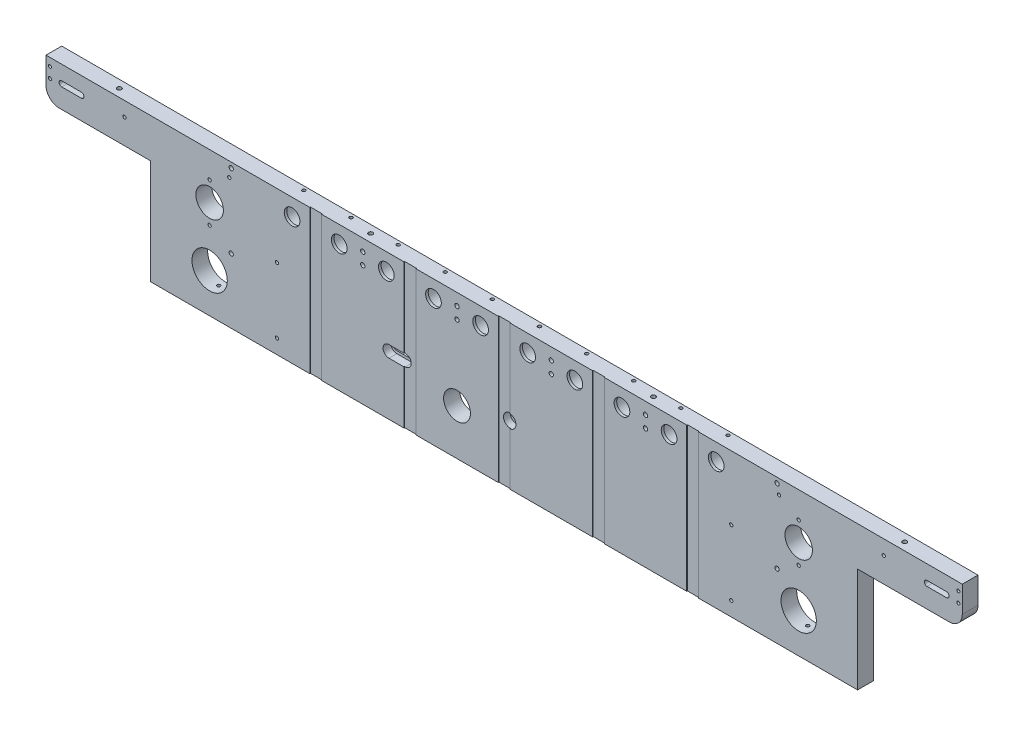
from build123d import *

# Parameters (mm, degrees)
EXTRUDE_1_DEPTH           = 12
FILLET_1_R                = 10
SKETCH_3_R                = 10.5
SKETCH_3_R_2              = 13.5
SKETCH_3_R_3              = 10.25
CUT_EXTRUDE_2_DEPTH       = 368.074924232
SKETCH_7_R                = 7.5
CUT_EXTRUDE_3_DEPTH       = 10
SKETCH_8_R                = 5.5
CUT_EXTRUDE_4_DEPTH       = 368.01498607
CUT_EXTRUDE_5_DEPTH       = 368.074924232
HOLE_WIZARD_M3_2_REACH    = 369.075
HOLE_WIZARD_M3_2_BORE_R   = 1.25
HOLE_WIZARD_M3_3_D        = 2.5
HOLE_WIZARD_1_D           = 5.5
HOLE_WIZARD_1_CBORE_D     = 10
HOLE_WIZARD_1_CBORE_DEPTH = 5.7
CUT_EXTRUDE_7_DEPTH       = 368.074924265
CUT_EXTRUDE_8_DEPTH       = 6
SKETCH_35_W               = 9
SKETCH_35_H               = 0.5
CUT_EXTRUDE_9_DEPTH       = 368.074924265
HOLE_WIZARD_M4_2_D        = 3.3
HOLE_WIZARD_M4_2_DEPTH    = 12
HOLE_WIZARD_M4_2_TIP      = 0.991420021
HOLE_WIZARD_M3_4_REACH    = 369.075
HOLE_WIZARD_M3_4_BORE_R   = 1.25
HOLE_WIZARD_M3_5_D        = 2.5
HOLE_WIZARD_M4_3_D        = 3.3
PATTERN_LINEAR_1_COUNT    = 4
PATTERN_LINEAR_1_PITCH    = 72
HOLE_WIZARD_M4_4_D        = 3.3
HOLE_WIZARD_M4_4_DEPTH    = 12
HOLE_WIZARD_M4_4_TIP      = 0.991420021
HOLE_WIZARD_2_D           = 2.4
HOLE_WIZARD_2_CBORE_D     = 4.3
HOLE_WIZARD_2_CBORE_DEPTH = 2.3
HOLE_WIZARD_3_D           = 2.4
HOLE_WIZARD_3_CBORE_D     = 4.3
HOLE_WIZARD_3_CBORE_DEPTH = 2.3
HOLE_WIZARD_4_D           = 12
HOLE_WIZARD_4_CBORE_D     = 16
HOLE_WIZARD_4_CBORE_DEPTH = 10
HOLE_WIZARD_M3_6_D        = 2.5


with BuildPart() as part:
    # 草图1 → 凸台-拉伸1 (new body)
    with BuildSketch(Plane.XY):
        Polygon((-350, -30), (-270, -30), (-270, -110), (270, -110), (270, -30), (350, -30), (350, 0), (-350, 0), align=None)
    extrude(amount=EXTRUDE_1_DEPTH)

    # 圆角1
    fillet_1_edges = [part.edges().sort_by_distance(p)[0] for p in [
        (350, -30, 6),
        (-350, -30, 6),
    ]]
    fillet(fillet_1_edges, radius=FILLET_1_R)

    # 草图3 → 切除-拉伸2 (cut, through all)
    with BuildSketch(Plane(origin=(0, 0, 0), x_dir=(-1, 0, 0), z_dir=(0, 0, -1))):
        with Locations((-225, -35)):
            Circle(SKETCH_3_R)
        with Locations((-225, -80)):
            Circle(SKETCH_3_R_2)
        with Locations(Location((225, -80, 0), (0, 0, 180))):
            Circle(SKETCH_3_R_2)
        with Locations(Location((225, -35, 0), (0, 0, 180))):
            Circle(SKETCH_3_R)
        with Locations((36, -75)):
            Circle(SKETCH_3_R_3)
    extrude(amount=-CUT_EXTRUDE_2_DEPTH, mode=Mode.SUBTRACT)

    # 草图7 → 切除-拉伸3 (cut)
    with BuildSketch(Plane(origin=(0, 0, 0), x_dir=(-1, 0, 0), z_dir=(0, 0, -1))):
        with Locations((-162, -13)):
            Circle(SKETCH_7_R)
        with Locations((-126, -13)):
            Circle(SKETCH_7_R)
        with Locations((-90, -13)):
            Circle(SKETCH_7_R)
        with Locations((-54, -13)):
            Circle(SKETCH_7_R)
        with Locations((-18, -13)):
            Circle(SKETCH_7_R)
        with Locations((18, -13)):
            Circle(SKETCH_7_R)
        with Locations((54, -13)):
            Circle(SKETCH_7_R)
        with Locations((90, -13)):
            Circle(SKETCH_7_R)
        with Locations((126, -13)):
            Circle(SKETCH_7_R)
        with Locations((162, -13)):
            Circle(SKETCH_7_R)
    extrude(amount=-CUT_EXTRUDE_3_DEPTH, mode=Mode.SUBTRACT)

    # 草图8 → 切除-拉伸4 (cut, through all)
    with BuildSketch(Plane(origin=(0, 0, 10), x_dir=(-1, 0, 0), z_dir=(0, 0, -1))):
        with Locations((-162, -13)):
            Circle(SKETCH_8_R)
        with Locations((-126, -13)):
            Circle(SKETCH_8_R)
        with Locations((-90, -13)):
            Circle(SKETCH_8_R)
        with Locations((-54, -13)):
            Circle(SKETCH_8_R)
        with Locations((-18, -13)):
            Circle(SKETCH_8_R)
        with Locations((18, -13)):
            Circle(SKETCH_8_R)
        with Locations((54, -13)):
            Circle(SKETCH_8_R)
        with Locations((90, -13)):
            Circle(SKETCH_8_R)
        with Locations((126, -13)):
            Circle(SKETCH_8_R)
        with Locations((162, -13)):
            Circle(SKETCH_8_R)
    extrude(amount=-CUT_EXTRUDE_4_DEPTH, mode=Mode.SUBTRACT)

    # 草图9 → 切除-拉伸5 (cut, through all)
    with BuildSketch(Plane(origin=(0, 0, 0), x_dir=(-1, 0, 0), z_dir=(0, 0, -1))):
        with BuildLine():
            Line((-338, -11), (-323, -11))
            ThreePointArc((-323, -11), (-321, -13), (-323, -15))
            Line((-323, -15), (-338, -15))
            ThreePointArc((-338, -15), (-340, -13), (-338, -11))
        make_face()
        with BuildLine():
            Line((338, -11), (323, -11))
            ThreePointArc((323, -11), (321, -13), (323, -15))
            Line((323, -15), (338, -15))
            ThreePointArc((338, -15), (340, -13), (338, -11))
        make_face()
    extrude(amount=-CUT_EXTRUDE_5_DEPTH, mode=Mode.SUBTRACT)

    # M3 螺纹孔2 bore → M3 螺纹孔2 (cut, up to next)
    with BuildSketch(Plane(origin=(0, -110, 0), x_dir=(-1, 0, 0), z_dir=(0, -1, 0)), mode=Mode.PRIVATE) as hole_wizard_m3_2_sk1:
        with Locations((225, -5)):
            Circle(HOLE_WIZARD_M3_2_BORE_R)
    hole_wizard_m3_2_tool1 = extrude(hole_wizard_m3_2_sk1.sketch, amount=-HOLE_WIZARD_M3_2_REACH, mode=Mode.PRIVATE) & part.part
    # M3 螺纹孔2 bore → M3 螺纹孔2 (cut, up to next)
    with BuildSketch(Plane(origin=(0, -110, 0), x_dir=(-1, 0, 0), z_dir=(0, -1, 0)), mode=Mode.PRIVATE) as hole_wizard_m3_2_sk2:
        with Locations((-225, -5)):
            Circle(HOLE_WIZARD_M3_2_BORE_R)
    hole_wizard_m3_2_tool2 = extrude(hole_wizard_m3_2_sk2.sketch, amount=-HOLE_WIZARD_M3_2_REACH, mode=Mode.PRIVATE) & part.part
    add(hole_wizard_m3_2_tool1.solids().sort_by_distance((-225, -110, 5))[0], mode=Mode.SUBTRACT)
    add(hole_wizard_m3_2_tool2.solids().sort_by_distance((225, -110, 5))[0], mode=Mode.SUBTRACT)

    # M3 螺纹孔3 (through all)
    with Locations(Plane.XY.offset(12)):
        with Locations((290, -11), (210, -11), (-210, -11), (-290, -11)):
            Hole(HOLE_WIZARD_M3_3_D / 2)

    # 打孔尺寸根据内六角圆柱头螺钉的类型1 (through all)
    with Locations(Plane.XY.offset(12)):
        with Locations((4, -65)):
            CounterBoreHole(HOLE_WIZARD_1_D / 2, HOLE_WIZARD_1_CBORE_D / 2, HOLE_WIZARD_1_CBORE_DEPTH)

    # 草图31 → 切除-拉伸7 (cut, through all)
    with BuildSketch(Plane.XY.offset(12)):
        with BuildLine():
            Line((-76, -67.5), (-88, -67.5))
            ThreePointArc((-88, -67.5), (-90.5, -65), (-88, -62.5))
            Line((-88, -62.5), (-76, -62.5))
            ThreePointArc((-76, -62.5), (-73.5, -65), (-76, -67.5))
        make_face()
    extrude(amount=-CUT_EXTRUDE_7_DEPTH, mode=Mode.SUBTRACT)

    # 草图32 → 切除-拉伸8 (cut)
    with BuildSketch(Plane.XY.offset(12)):
        with BuildLine():
            Line((-88, -60.5), (-76, -60.5))
            ThreePointArc((-76, -60.5), (-71.5, -65), (-76, -69.5))
            Line((-76, -69.5), (-88, -69.5))
            ThreePointArc((-88, -69.5), (-92.5, -65), (-88, -60.5))
        make_face()
    extrude(amount=-CUT_EXTRUDE_8_DEPTH, mode=Mode.SUBTRACT)

    # 草图35 → 切除-拉伸9 (cut, through all)
    with BuildSketch(Plane(origin=(0, 0, 0), x_dir=(1, 0, 0), z_dir=(0, 1, 0))):
        with Locations((-144, -11.75)):
            Rectangle(SKETCH_35_W, SKETCH_35_H)
        with Locations((-72, -11.75)):
            Rectangle(SKETCH_35_W, SKETCH_35_H)
        with Locations((0, -11.75)):
            Rectangle(SKETCH_35_W, SKETCH_35_H)
        with Locations((72, -11.75)):
            Rectangle(SKETCH_35_W, SKETCH_35_H)
        with Locations((144, -11.75)):
            Rectangle(SKETCH_35_W, SKETCH_35_H)
    extrude(amount=-CUT_EXTRUDE_9_DEPTH, mode=Mode.SUBTRACT)

    # M4 螺纹孔2
    with Locations(Plane(origin=(0, 0, 0), x_dir=(1, 0, 0), z_dir=(0, 1, 0))):
        with Locations((300, -6), (108, -6), (-108, -6), (-300, -6)):
            Hole(HOLE_WIZARD_M4_2_D / 2, depth=HOLE_WIZARD_M4_2_DEPTH)
            with Locations((0, 0, -(HOLE_WIZARD_M4_2_DEPTH + HOLE_WIZARD_M4_2_TIP / 2))):  # 118° drill point
                Cone(0, HOLE_WIZARD_M4_2_D / 2, HOLE_WIZARD_M4_2_TIP, mode=Mode.SUBTRACT)

    # M3 螺纹孔4 bore → M3 螺纹孔4 (cut, up to next)
    with BuildSketch(Plane(origin=(0, 0, 0), x_dir=(1, 0, 0), z_dir=(0, 1, 0)), mode=Mode.PRIVATE) as hole_wizard_m3_4_sk1:
        with Locations((-162, -3)):
            Circle(HOLE_WIZARD_M3_4_BORE_R)
    hole_wizard_m3_4_tool1 = extrude(hole_wizard_m3_4_sk1.sketch, amount=-HOLE_WIZARD_M3_4_REACH, mode=Mode.PRIVATE) & part.part
    # M3 螺纹孔4 bore → M3 螺纹孔4 (cut, up to next)
    with BuildSketch(Plane(origin=(0, 0, 0), x_dir=(1, 0, 0), z_dir=(0, 1, 0)), mode=Mode.PRIVATE) as hole_wizard_m3_4_sk2:
        with Locations((-126, -3)):
            Circle(HOLE_WIZARD_M3_4_BORE_R)
    hole_wizard_m3_4_tool2 = extrude(hole_wizard_m3_4_sk2.sketch, amount=-HOLE_WIZARD_M3_4_REACH, mode=Mode.PRIVATE) & part.part
    # M3 螺纹孔4 bore → M3 螺纹孔4 (cut, up to next)
    with BuildSketch(Plane(origin=(0, 0, 0), x_dir=(1, 0, 0), z_dir=(0, 1, 0)), mode=Mode.PRIVATE) as hole_wizard_m3_4_sk3:
        with Locations((-90, -3)):
            Circle(HOLE_WIZARD_M3_4_BORE_R)
    hole_wizard_m3_4_tool3 = extrude(hole_wizard_m3_4_sk3.sketch, amount=-HOLE_WIZARD_M3_4_REACH, mode=Mode.PRIVATE) & part.part
    # M3 螺纹孔4 bore → M3 螺纹孔4 (cut, up to next)
    with BuildSketch(Plane(origin=(0, 0, 0), x_dir=(1, 0, 0), z_dir=(0, 1, 0)), mode=Mode.PRIVATE) as hole_wizard_m3_4_sk4:
        with Locations((-54, -3)):
            Circle(HOLE_WIZARD_M3_4_BORE_R)
    hole_wizard_m3_4_tool4 = extrude(hole_wizard_m3_4_sk4.sketch, amount=-HOLE_WIZARD_M3_4_REACH, mode=Mode.PRIVATE) & part.part
    # M3 螺纹孔4 bore → M3 螺纹孔4 (cut, up to next)
    with BuildSketch(Plane(origin=(0, 0, 0), x_dir=(1, 0, 0), z_dir=(0, 1, 0)), mode=Mode.PRIVATE) as hole_wizard_m3_4_sk5:
        with Locations((-18, -3)):
            Circle(HOLE_WIZARD_M3_4_BORE_R)
    hole_wizard_m3_4_tool5 = extrude(hole_wizard_m3_4_sk5.sketch, amount=-HOLE_WIZARD_M3_4_REACH, mode=Mode.PRIVATE) & part.part
    # M3 螺纹孔4 bore → M3 螺纹孔4 (cut, up to next)
    with BuildSketch(Plane(origin=(0, 0, 0), x_dir=(1, 0, 0), z_dir=(0, 1, 0)), mode=Mode.PRIVATE) as hole_wizard_m3_4_sk6:
        with Locations((18, -3)):
            Circle(HOLE_WIZARD_M3_4_BORE_R)
    hole_wizard_m3_4_tool6 = extrude(hole_wizard_m3_4_sk6.sketch, amount=-HOLE_WIZARD_M3_4_REACH, mode=Mode.PRIVATE) & part.part
    # M3 螺纹孔4 bore → M3 螺纹孔4 (cut, up to next)
    with BuildSketch(Plane(origin=(0, 0, 0), x_dir=(1, 0, 0), z_dir=(0, 1, 0)), mode=Mode.PRIVATE) as hole_wizard_m3_4_sk7:
        with Locations((54, -3)):
            Circle(HOLE_WIZARD_M3_4_BORE_R)
    hole_wizard_m3_4_tool7 = extrude(hole_wizard_m3_4_sk7.sketch, amount=-HOLE_WIZARD_M3_4_REACH, mode=Mode.PRIVATE) & part.part
    # M3 螺纹孔4 bore → M3 螺纹孔4 (cut, up to next)
    with BuildSketch(Plane(origin=(0, 0, 0), x_dir=(1, 0, 0), z_dir=(0, 1, 0)), mode=Mode.PRIVATE) as hole_wizard_m3_4_sk8:
        with Locations((90, -3)):
            Circle(HOLE_WIZARD_M3_4_BORE_R)
    hole_wizard_m3_4_tool8 = extrude(hole_wizard_m3_4_sk8.sketch, amount=-HOLE_WIZARD_M3_4_REACH, mode=Mode.PRIVATE) & part.part
    # M3 螺纹孔4 bore → M3 螺纹孔4 (cut, up to next)
    with BuildSketch(Plane(origin=(0, 0, 0), x_dir=(1, 0, 0), z_dir=(0, 1, 0)), mode=Mode.PRIVATE) as hole_wizard_m3_4_sk9:
        with Locations((126, -3)):
            Circle(HOLE_WIZARD_M3_4_BORE_R)
    hole_wizard_m3_4_tool9 = extrude(hole_wizard_m3_4_sk9.sketch, amount=-HOLE_WIZARD_M3_4_REACH, mode=Mode.PRIVATE) & part.part
    # M3 螺纹孔4 bore → M3 螺纹孔4 (cut, up to next)
    with BuildSketch(Plane(origin=(0, 0, 0), x_dir=(1, 0, 0), z_dir=(0, 1, 0)), mode=Mode.PRIVATE) as hole_wizard_m3_4_sk10:
        with Locations((162, -3)):
            Circle(HOLE_WIZARD_M3_4_BORE_R)
    hole_wizard_m3_4_tool10 = extrude(hole_wizard_m3_4_sk10.sketch, amount=-HOLE_WIZARD_M3_4_REACH, mode=Mode.PRIVATE) & part.part
    add(hole_wizard_m3_4_tool1.solids().sort_by_distance((-162, 0, 3))[0], mode=Mode.SUBTRACT)
    add(hole_wizard_m3_4_tool2.solids().sort_by_distance((-126, 0, 3))[0], mode=Mode.SUBTRACT)
    add(hole_wizard_m3_4_tool3.solids().sort_by_distance((-90, 0, 3))[0], mode=Mode.SUBTRACT)
    add(hole_wizard_m3_4_tool4.solids().sort_by_distance((-54, 0, 3))[0], mode=Mode.SUBTRACT)
    add(hole_wizard_m3_4_tool5.solids().sort_by_distance((-18, 0, 3))[0], mode=Mode.SUBTRACT)
    add(hole_wizard_m3_4_tool6.solids().sort_by_distance((18, 0, 3))[0], mode=Mode.SUBTRACT)
    add(hole_wizard_m3_4_tool7.solids().sort_by_distance((54, 0, 3))[0], mode=Mode.SUBTRACT)
    add(hole_wizard_m3_4_tool8.solids().sort_by_distance((90, 0, 3))[0], mode=Mode.SUBTRACT)
    add(hole_wizard_m3_4_tool9.solids().sort_by_distance((126, 0, 3))[0], mode=Mode.SUBTRACT)
    add(hole_wizard_m3_4_tool10.solids().sort_by_distance((162, 0, 3))[0], mode=Mode.SUBTRACT)

    # M3 螺纹孔5 (through all)
    with Locations(Plane(origin=(0, 0, 0), x_dir=(-1, 0, 0), z_dir=(0, 0, -1))):
        with Locations((-173.5, -49), (-173.5, -99), (173.5, -49), (173.5, -99)):
            Hole(HOLE_WIZARD_M3_5_D / 2)

    # M4 螺纹孔3 (through all)
    with Locations(Plane(origin=(0, 0, 0), x_dir=(-1, 0, 0), z_dir=(0, 0, -1))):
        with Locations((-108, -9), (-108, -18)):
            hole_wizard_m4_3 = Hole(HOLE_WIZARD_M4_3_D / 2)

    # 阵列(线性)1: M4 螺纹孔3 ×4
    with Locations(*[(-i * PATTERN_LINEAR_1_PITCH, 0, 0) for i in range(1, PATTERN_LINEAR_1_COUNT)]):
        add(hole_wizard_m4_3, mode=Mode.SUBTRACT)

    # M4 螺纹孔4
    with Locations(Plane(origin=(0, 0, 0), x_dir=(-1, 0, 0), z_dir=(0, 0, -1))):
        with Locations((208.5, -60.5), (208.5, -4), (-208.5, -60.5), (-208.5, -4)):
            Hole(HOLE_WIZARD_M4_4_D / 2, depth=HOLE_WIZARD_M4_4_DEPTH)
            with Locations((0, 0, -(HOLE_WIZARD_M4_4_DEPTH + HOLE_WIZARD_M4_4_TIP / 2))):  # 118° drill point
                Cone(0, HOLE_WIZARD_M4_4_D / 2, HOLE_WIZARD_M4_4_TIP, mode=Mode.SUBTRACT)

    # 打孔尺寸根据内六角圆柱头螺钉的类型2 (through all)
    with Locations(Plane(origin=(0, 0, 0), x_dir=(-1, 0, 0), z_dir=(0, 0, -1))):
        with Locations((347, -6), (347, -14)):
            CounterBoreHole(HOLE_WIZARD_2_D / 2, HOLE_WIZARD_2_CBORE_D / 2, HOLE_WIZARD_2_CBORE_DEPTH)

    # 打孔尺寸根据内六角圆柱头螺钉的类型3 (through all)
    with Locations(Plane(origin=(0, 0, 0), x_dir=(-1, 0, 0), z_dir=(0, 0, -1))):
        with Locations((-347, -6), (-347, -14)):
            CounterBoreHole(HOLE_WIZARD_3_D / 2, HOLE_WIZARD_3_CBORE_D / 2, HOLE_WIZARD_3_CBORE_DEPTH)

    # 打孔尺寸根据内六角圆柱头螺钉的类型4 (through all)
    with Locations(Plane(origin=(0, 0, 0), x_dir=(-1, 0, 0), z_dir=(0, 0, -1))):
        with Locations((-162, -13), (-126, -13), (-90, -13), (-54, -13), (-18, -13), (18, -13), (54, -13), (90, -13), (126, -13), (162, -13)):
            CounterBoreHole(HOLE_WIZARD_4_D / 2, HOLE_WIZARD_4_CBORE_D / 2, HOLE_WIZARD_4_CBORE_DEPTH)

    # M3 螺纹孔6 (through all)
    with Locations(Plane(origin=(0, 0, 0), x_dir=(-1, 0, 0), z_dir=(0, 0, -1))):
        with Locations((225, -50), (225, -20), (-225, -20), (-225, -50)):
            Hole(HOLE_WIZARD_M3_6_D / 2)


solid = part.part
